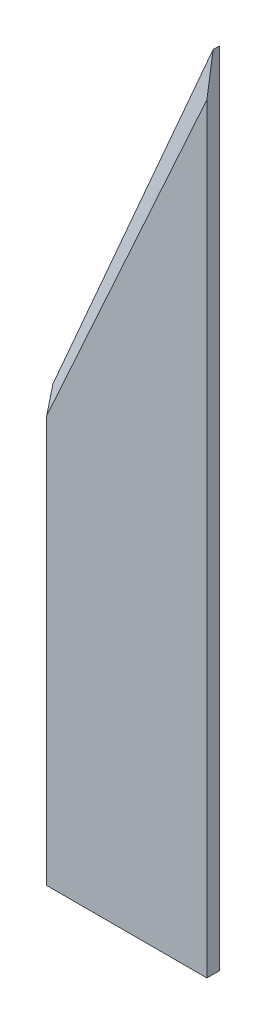
from build123d import *

# Parameters (mm, degrees)
SKETCH1_W           = 13
SKETCH1_H           = 1
BOSS_EXTRUDE1_DEPTH = 35
CUT_EXTRUDE2_DEPTH  = 36.612497806
SKETCH8_W           = 13
SKETCH8_H           = 1
BOSS_EXTRUDE2_DEPTH = 30


with BuildPart() as part:
    # Sketch1 → Boss-Extrude1 (new body)
    with BuildSketch(Plane(origin=(0, 0, 0), x_dir=(1, 0, 0), z_dir=(0, 1, 0))):
        Rectangle(SKETCH1_W, SKETCH1_H)
    extrude(amount=BOSS_EXTRUDE1_DEPTH)

    # Sketch3 → Cut-Extrude2 (cut, through all)
    with BuildSketch(Plane.XY.offset(0.5)):
        Polygon((6.5, 35), (-6.5, 5), (-6.5, 35), align=None)
    extrude(amount=-CUT_EXTRUDE2_DEPTH, mode=Mode.SUBTRACT)

    # Sketch7 → Cut-Loft2 section 0
    with BuildSketch(Plane(origin=(6.5, 0, 0), x_dir=(0, 0, -1), z_dir=(1, 0, 0))):
        with BuildLine():
            Line((0, 35), (-0.5, 31.730868962))
            Line((-0.5, 31.730868962), (-0.5, 35))
            Line((-0.5, 35), (0, 35))
        make_face()
    # Sketch6 → Cut-Loft2 section 1
    with BuildSketch(Plane.ZY.offset(6.5)):
        with BuildLine():
            Line((0, 5), (0.5, 3.027523124))
            Line((0.5, 3.027523124), (0.5, 5))
            Line((0.5, 5), (0, 5))
        make_face()
    loft(mode=Mode.SUBTRACT)

    # Sketch8 → Boss-Extrude2 (add)
    with BuildSketch(Plane.XZ):
        Rectangle(SKETCH8_W, SKETCH8_H)
    extrude(amount=BOSS_EXTRUDE2_DEPTH)


solid = part.part
